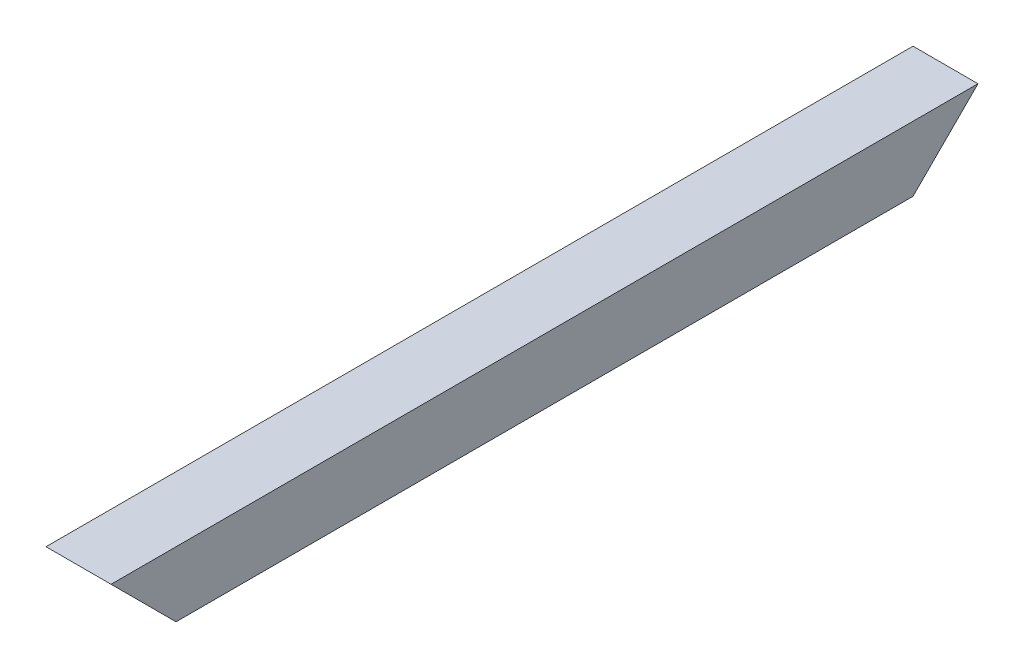
SolidWorks part; units mm, degrees
ref_plane "Front Plane" through (0, 0, 0) normal (0, 0, 1) x (1, 0, 0)
ref_plane "Top Plane" through (0, 0, 0) normal (0, 1, 0) x (1, 0, 0)
ref_plane "Right Plane" through (0, 0, 0) normal (1, 0, 0) x (0, 0, -1)
other "Configuration Table"
sketch "Sketch1" plane through (0, 0, 0) normal (0, 0, 1) x (1, 0, 0)
  line L0 (-45.1417, 25.901) -> (-15.1417, 25.901)
  line L1 (-15.1417, 25.901) -> (-15.1417, -4.099)
  line L2 (-15.1417, -4.099) -> (-45.1417, -4.099)
  line L3 (-45.1417, -4.099) -> (-45.1417, 25.901)
extrude "Boss-Extrude1" add sketch "Sketch1" along normal blind 400
sketch "Sketch2" plane through (0, 0, 400) normal (0, 0, 1) x (1, 0, 0)
  line L0 (-42.1417, 22.901) -> (-18.1417, 22.901)
  line L1 (-18.1417, 22.901) -> (-18.1417, -1.099)
  line L2 (-18.1417, -1.099) -> (-42.1417, -1.099)
  line L3 (-42.1417, -1.099) -> (-42.1417, 22.901)
  line L4 (-15.1417, -4.099) -> (-15.1417, 25.901) construction
  line L5 (-15.1417, 25.901) -> (-45.1417, 25.901) construction
  line L6 (-45.1417, 25.901) -> (-45.1417, -4.099) construction
  line L7 (-45.1417, -4.099) -> (-15.1417, -4.099) construction
  dimension "D1" = 3
  dimension "D2" = 3
  dimension "D3" = 3
  dimension "D4" = 3
extrude "Cut-Extrude1" cut sketch "Sketch2" against normal blind 492
sketch "Sketch4" plane through (-15.1417, 0, 0) normal (1, 0, 0) x (0, 0, -1)
  line L0 (0, 25.901) -> (-30, -4.099)
  line L1 (-400, -4.099) -> (0, -4.099) construction
  line L2 (-30, -4.099) -> (0, -4.099)
  line L3 (0, -4.099) -> (0, 25.901)
  dimension "D1" = 45
extrude "Cut-Extrude3" cut sketch "Sketch4" against normal through all
sketch "Sketch8" plane through (-15.1417, 0, 0) normal (1, 0, 0) x (0, 0, -1)
  line L0 (-400, 25.901) -> (-370, -4.099)
  line L1 (-400, -4.099) -> (-30, -4.099) construction
  line L2 (-370, -4.099) -> (-400, -4.099)
  line L3 (-400, -4.099) -> (-400, 25.901)
  dimension "D1" = 45
extrude "Cut-Extrude6" cut sketch "Sketch8" against normal through all
